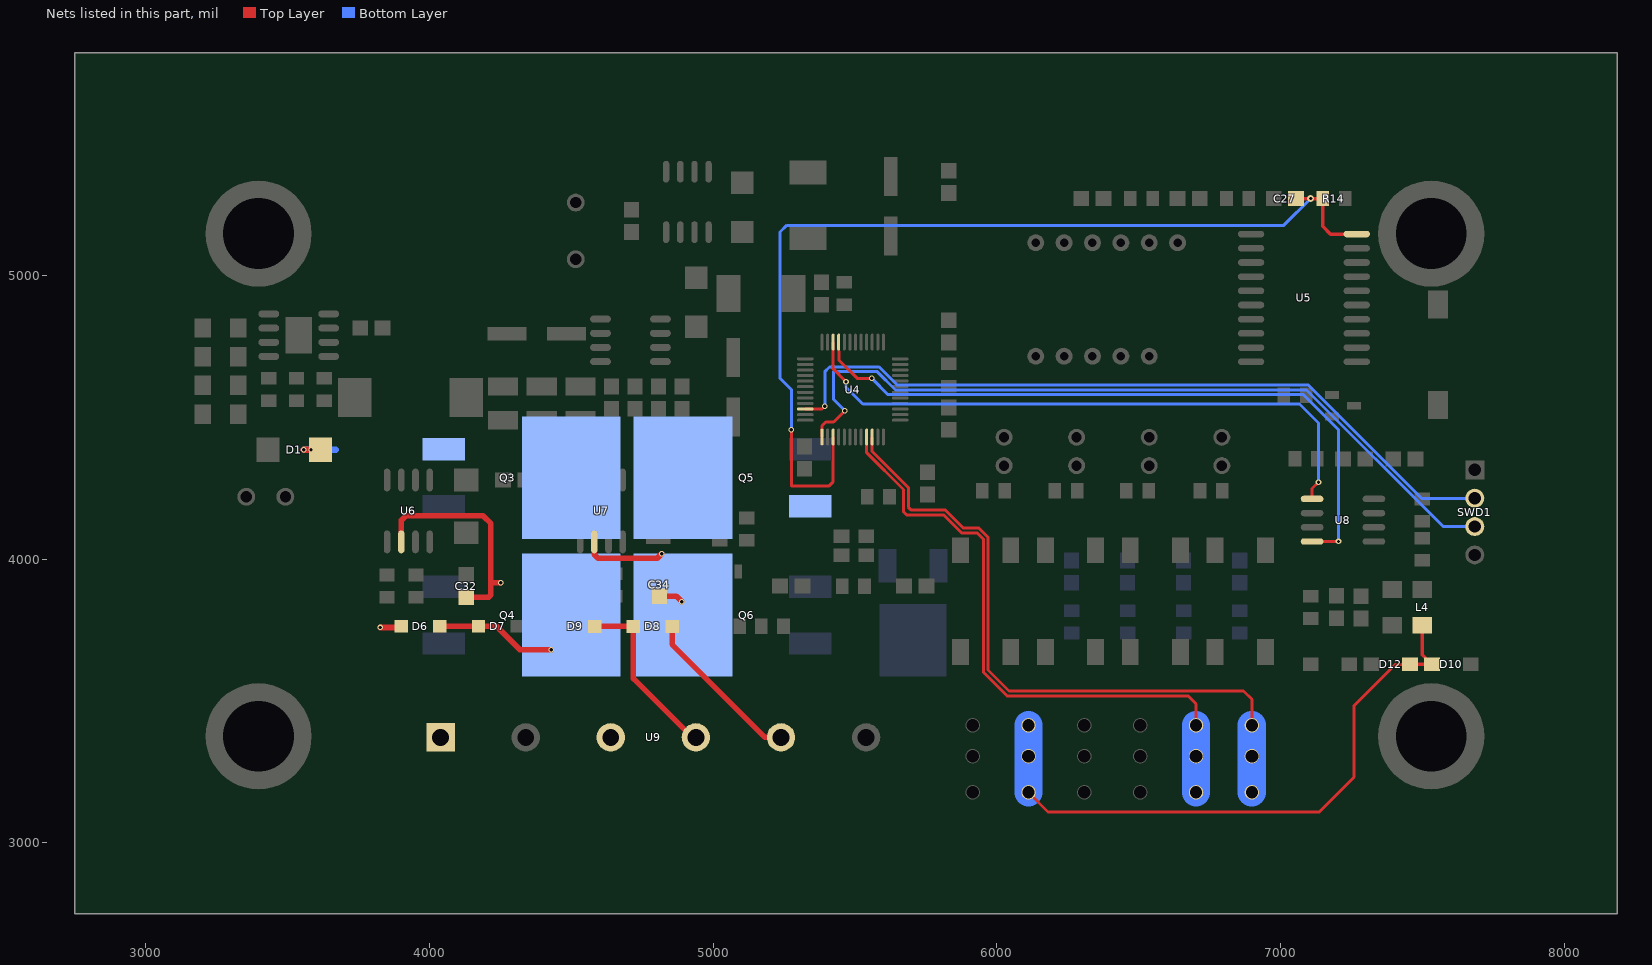
[diagram p0: the nets of this part, all layers, seen from the top]
# Altium PCB MISC82093.pcbdoc (part 2 of 2)
Units mil, origin at the board's own origin, x right, y up, seen from the top; angles counter-clockwise.
Board outline 5437 x 3035.4 mil, 2 copper layers (Top Layer, Bottom Layer), stack 62.2 mil thick; 117 components, 84 nets, 389 pads, 166 vias.

## Via types
v1: diameter 19.7, hole 11.8, Top Layer to Bottom Layer, 157 vias
v2: diameter 24, hole 12, Top Layer to Bottom Layer, 9 vias

## Nets (pads, with @x,y where several pads share a name; then routed paths per layer and width w, separated by ;. In a path a pad name is that pad's centre, name@x,y a point inside that pad or via, vN(x,y) a via of type N, cw(c..) or ccw(c..) an arc to the next point about the centre after c; other vN are vias at no path point) (continued)
RS485-B: D10.1 D12.2 L4.2 pad.0@6111.9,3178.4 pad.0@6111.9,3414.6 pad.2 | length 2202.3
  Top Layer w10.6: pad.0@6111.9,3178.4 6180.9,3109.4 7136.8,3109.4 7259.5,3232.1 7259.5,3483.9 7405.5,3629.9 D12.2@7456.8,3629.9
  Top Layer w12.5: D12.2@7456.8,3629.9 D10.1@7534.1,3629.9 7500,3664 L4.2@7500,3768
  Bottom Layer w100: pad.0@6111.9,3178.4 pad.2@6111.9,3305.9 pad.0@6111.9,3414.6
RXD: U4.22 U8.1 | length 2172.7
  Top Layer w10.6: U4.22@5423.2,4765.7 5423.2,4671.3 v1(5468.5,4626) ; U8.1@7111.5,4212.8 7111.5,4249.2 v1(7134,4271.7)
  Bottom Layer w10.6: v1(5468.5,4626) 5468.5,4606.3 5527.6,4547.2 7067.1,4547.2 7134,4480.4 v1(7134,4271.7)
S1: pad.0@6702.4,3178.4 pad.0@6702.4,3414.6 pad.3@6702.4,3305.9 U4.45 | length 2215.6
  Top Layer w10.6: U4.45@5541.3,4431.1 5541.3,4376 5671.5,4245.9 5671.5,4167.2 5682.1,4156.6 5812.5,4156.6 5876,4093.1 5930.6,4093.1 5952.5,4071.2 5952.5,3602.7 6036.4,3518.8 6674.1,3518.8 6702.4,3490.5 pad.0@6702.4,3414.6
  Bottom Layer w100: pad.0@6702.4,3178.4 pad.3@6702.4,3305.9 pad.0@6702.4,3414.6
S2: pad.0@6899.3,3178.4 pad.0@6899.3,3414.6 pad.4@6899.3,3305.9 U4.46 | length 2394
  Top Layer w10.6: U4.46@5561,4431.1 5561,4379.8 5688.1,4252.7 5688.1,4183.9 5698.7,4173.2 5819.4,4173.2 5882.9,4109.8 5937.5,4109.8 5969.2,4078.1 5969.2,3609.6 6043.3,3535.4 6870.1,3535.4 6899.3,3506.2 pad.0@6899.3,3414.6
  Bottom Layer w100: pad.0@6899.3,3178.4 pad.4@6899.3,3305.9 pad.0@6899.3,3414.6
STB: C27.1 R14.1 U4.39 U5.20 | length 3464.8
  Top Layer w10.6: v1(5275.6,4456.7) 5275.6,4259.8 5277.8,4257.7 5407.3,4257.7 5423.2,4273.6 U4.39@5423.2,4431.1
  Top Layer w12.5: C27.1@7055.1,5271.7 v2(7106.3,5271.7) R14.1@7149.2,5271.7 7149.2,5173.6 7176.6,5146.3 U5.20@7268.9,5146.3
  Bottom Layer w10.6: v1(5275.6,4456.7) 5275.6,4598.4 5236.2,4637.8 5236.2,5153.5 5259.8,5177.2 7011.8,5177.2 v2(7106.3,5271.7)
SWCLK: SWD1.3 U4.37 | length 2782.1
  Top Layer w10.6: U4.37@5383.9,4431.1 5383.9,4470.5 5397.6,4484.3 5425.2,4484.3 v1(5464.6,4523.6)
  Bottom Layer w10.6: v1(5464.6,4523.6) 5425.2,4563 5425.2,4661.4 5578.7,4661.4 5643,4597.1 7091.8,4597.1 7573.6,4115.4 SWD1.3@7685,4115.4
SWDIO: SWD1.2 U4.34 | length 2686.4
  Top Layer w10.6: U4.34@5324.8,4529.5 5383.9,4529.5 v1(5393.7,4539.4)
  Bottom Layer w10.6: v1(5393.7,4539.4) 5393.7,4661.4 5410.3,4678 5585.6,4678 5649.9,4613.8 7098.7,4613.8 7499,4213.5 7683.2,4213.5 SWD1.2@7685,4215.4
T+: C32.1 D6.2 D7.1 Q3.3 Q4.4 U6.6 U9.3 | length 1215.2
  Top Layer w20: U6.6@3900.9,4061.2 3900.9,4137.1 3917.3,4153.5 4189,4153.5 4216.5,4126 4216.5,3913.4 ; D6.2@4036.8,3763.8 D7.1@4173.2,3763.8 4236.2,3763.8 4318.9,3681.1 v1(4429.1,3681.1) ; C32.1@4129.9,3866.1 4208.7,3866.1 4216.5,3874 4216.5,3913.4 ; v1(4252,3917.3) 4220.5,3917.3 4216.5,3913.4
T-: C34.1 D8.2 D9.1 Q5.3 Q6.4 U7.6 U9.4 | length 1006.9
  Top Layer w20: U7.6@4581.3,4061.2 4581.3,4017.1 4594.5,4003.9 4803.1,4003.9 v1(4818.9,4019.7) ; D9.1@4582.7,3763.5 D8.2@4719.1,3763.5 4719.1,3580.1 4927,3372.2 U9.4@4939.4,3372.2 ; C34.1@4811,3870.1 4870.1,3870.1 v1(4889.8,3850.4)
TXD: U4.21 U8.4 | length 2413.6
  Top Layer w10.6: U4.21@5442.9,4765.7 5443,4702.7 5507.9,4637.8 v1(5559.1,4637.8) ; U8.4@7111.5,4062.8 7111.7,4063 v1(7204.7,4063)
  Bottom Layer w10.6: v1(5559.1,4637.8) 5616.3,4580.5 7080.9,4580.5 7204.7,4456.7 v1(7204.7,4063)
VCC: D1.2 D6.1 D8.1 Q3.4 Q5.4 U9.1 U9.5 | length 847.6
  Top Layer w20: v1(3826.8,3759.8) 3896.3,3759.8 D6.1@3900.2,3763.8 ; D8.1@4855.7,3763.5 4855.7,3699.4 5182.9,3372.2 U9.5@5239.4,3372.2
  Top Layer w23.6: v1(3557,4385.8) v1(3582.8,4385.8) D1.2@3633.9,4385.8
  Bottom Layer w23.6: v1(3557,4385.8) v1(3582.8,4385.8) 3669.3,4385.8
pads on no net: SW1.2 SW2.2 SW3.2 SW4.2 U1.6 U4.2 U4.3 U4.4 U4.19 U4.25 U4.26 U4.29 U4.33 U4.38 U5.10 U5.11 U5.13
copper on no net:
  other v1: 3366.2,3228.4 3429,3228.4 7500.1,3228.4 7562.9,3228.4 3308.9,3254 3486.4,3254 7442.7,3254 7620.3,3254 3266.9,3300.6 3528.4,3300.6 7400.7,3300.6 7662.3,3300.6 3247.5,3360.4 3547.8,3360.4 7381.3,3360.4 7681.7,3360.4 3254,3422.8 3541.3,3422.8 7387.9,3422.8 7675.1,3422.8 3285.4,3477.2 3509.9,3477.2 7419.3,3477.2 7643.7,3477.2 3336.2,3514.1 3459.1,3514.1 7470.1,3514.1 7592.9,3514.1 3397.6,3527.1 7531.5,3527.1 3366.2,5000.1 3429,5000.1 7500.1,5000.1 7562.9,5000.1 3308.9,5025.6 3486.4,5025.6 7442.7,5025.6 7620.3,5025.6 3266.9,5072.3 3528.4,5072.3 7400.7,5072.3 7662.3,5072.3 3247.5,5132 3547.8,5132 7381.3,5132 7681.7,5132 3254,5194.5 3541.3,5194.5 7387.9,5194.5 7675.1,5194.5 3285.4,5248.8 3509.9,5248.8 7419.3,5248.8 7643.7,5248.8 3336.2,5285.7 3459.1,5285.7 7470.1,5285.7 7592.9,5285.7 3397.6,5298.8 7531.5,5298.8

## Polygon pours and split planes (outlines as drawn)
VCC on Top Layer (solid, remove dead copper, pour order 6): 4137.8,3543.3 4179.8,3501.3 4179.8,3100.6 4150.1,3070.9 3858.3,3070.9 3858.3,3543.3
GND on Top Layer (solid, remove dead copper, pour order 10): 3019.7,5523.6 3019.7,3000 7905.5,3000 7905.5,5523.6
VCC on Bottom Layer (solid, remove dead copper, pour order 24): 4317.2,4051.2 4281.8,4086.6 4281.8,4525.3 4267.7,4539.4 3908.6,4539.4 3874,4504.8 3874,3547.2 3913.4,3507.9 4137.8,3507.9 4161.4,3484.3 4161.4,3255.9 4133.9,3228.3 3641.7,3228.3 3618.1,3252 3618.1,4752 3673.2,4807.1 5070.9,4807.1 5110.2,4767.7 5110.2,4063 5098.4,4051.2
T+ on Bottom Layer (solid, remove dead copper, pour order 26): 4511.8,3232.3 4496.1,3248 4496.1,3468.5 4437,3527.6 4354.3,3527.6 4205.3,3676.6 4205.3,3987.3 4180.8,4011.8 3893.7,4011.8 3877.8,4027.7 3877.8,4504.8 3910.9,4537.9 4247.9,4537.9 4275.6,4510.2 4275.6,4080.4 4308.8,4047.2 4673.2,4047.2 4692.9,4027.6 4692.9,3559.1 4779.7,3472.2 4779.7,3250.2 4761.8,3232.3
T- on Bottom Layer (solid, remove dead copper, pour order 28): 4791.3,3468.5 4696.9,3563 4696.9,4031.5 4712.6,4047.2 5098.4,4047.2 5113.5,4062.3 5113.5,4148.9 5114.2,4149.6 5114.2,4259.8 5129.9,4275.6 5437.2,4275.6 5453,4259.8 5453,4008.1 5440.9,3996.1 5255.9,3996.1 5236.2,3976.4 5236.2,3645.7 5063,3472.4 5063,3252 5043.8,3232.8 4806.6,3232.8 4791.3,3248
VCC on Top Layer (solid, remove dead copper, pour order 8): 5102.4,3476.4 5326.8,3476.4 5358.3,3444.9 5358.3,3102.4 5334.6,3078.7 4141.7,3078.7 4118.1,3102.4 4118.1,3263.8 4145.7,3291.3 5051.2,3291.3 5078.7,3318.9 5078.7,3452.8
GND on Bottom Layer (solid, remove dead copper, pour order 30): 3000,5535.4 3000,3000 7937,3000 7937,5535.4

## Keep-outs
Top Layer:
  region: 3594.5,5147.8 3594.1,5135.3 3592.9,5122.9 3590.9,5110.5 3588.2,5098.4 3584.7,5086.4 3580.4,5074.6 3575.4,5063.2 3569.7,5052.1 3563.2,5041.4 3556.2,5031.1 3548.4,5021.3 3540.1,5012 3531.2,5003.2 3521.8,4995 3511.8,4987.4 3501.4,4980.5 3490.6,4974.3 3479.4,4968.7 3467.9,4963.9 3456.1,4959.8 3444,4956.5 3431.8,4953.9 3419.5,4952.2 3407,4951.2 3394.5,4951 3382,4951.6 3369.6,4952.9 3357.3,4955.1 3345.2,4958.1 3333.3,4961.8 3321.6,4966.2 3310.2,4971.4 3299.2,4977.3 3288.6,4983.9 3278.4,4991.1 3268.7,4999 3259.6,5007.5 3250.9,5016.5 3242.9,5026.1 3235.5,5036.2 3228.7,5046.7 3222.7,5057.6 3217.3,5068.9 3212.7,5080.5 3208.8,5092.3 3205.6,5104.4 3203.3,5116.7 3201.7,5129.1 3200.9,5141.5 3200.9,5154 3201.7,5166.5 3203.3,5178.9 3205.6,5191.2 3208.8,5203.3 3212.7,5215.1 3217.3,5226.7 3222.7,5238 3228.7,5248.9 3235.5,5259.4 3242.9,5269.5 3250.9,5279 3259.6,5288.1 3268.7,5296.6 3278.4,5304.4 3288.6,5311.7 3299.2,5318.3 3310.2,5324.2 3321.6,5329.4 3333.3,5333.8 3345.2,5337.5 3357.3,5340.5 3369.6,5342.6 3382,5344 3394.5,5344.6 3407,5344.4 3419.5,5343.4 3431.8,5341.7 3444,5339.1 3456.1,5335.8 3467.9,5331.7 3479.4,5326.9 3490.6,5321.3 3501.4,5315.1 3511.8,5308.1 3521.8,5300.6 3531.2,5292.4 3540.1,5283.6 3548.4,5274.3 3556.2,5264.5 3563.2,5254.2 3569.7,5243.5 3575.4,5232.4 3580.4,5221 3584.7,5209.2 3588.2,5197.2 3590.9,5185 3592.9,5172.7 3594.1,5160.3
  region: 3594.5,3376.1 3594.1,3363.7 3592.9,3351.2 3590.9,3338.9 3588.2,3326.7 3584.7,3314.7 3580.4,3303 3575.4,3291.5 3569.7,3280.4 3563.2,3269.7 3556.2,3259.4 3548.4,3249.6 3540.1,3240.3 3531.2,3231.5 3521.8,3223.4 3511.8,3215.8 3501.4,3208.9 3490.6,3202.6 3479.4,3197.1 3467.9,3192.3 3456.1,3188.2 3444,3184.8 3431.8,3182.3 3419.5,3180.5 3407,3179.5 3394.5,3179.3 3382,3179.9 3369.6,3181.3 3357.3,3183.5 3345.2,3186.4 3333.3,3190.1 3321.6,3194.6 3310.2,3199.8 3299.2,3205.7 3288.6,3212.3 3278.4,3219.5 3268.7,3227.4 3259.6,3235.8 3250.9,3244.9 3242.9,3254.5 3235.5,3264.5 3228.7,3275 3222.7,3285.9 3217.3,3297.2 3212.7,3308.8 3208.8,3320.7 3205.6,3332.8 3203.3,3345 3201.7,3357.4 3200.9,3369.9 3200.9,3382.4 3201.7,3394.9 3203.3,3407.2 3205.6,3419.5 3208.8,3431.6 3212.7,3443.5 3217.3,3455.1 3222.7,3466.3 3228.7,3477.3 3235.5,3487.8 3242.9,3497.8 3250.9,3507.4 3259.6,3516.4 3268.7,3524.9 3278.4,3532.8 3288.6,3540 3299.2,3546.6 3310.2,3552.5 3321.6,3557.7 3333.3,3562.2 3345.2,3565.9 3357.3,3568.8 3369.6,3571 3382,3572.4 3394.5,3573 3407,3572.8 3419.5,3571.8 3431.8,3570 3444,3567.4 3456.1,3564.1 3467.9,3560 3479.4,3555.2 3490.6,3549.7 3501.4,3543.4 3511.8,3536.5 3521.8,3528.9 3531.2,3520.7 3540.1,3512 3548.4,3502.7 3556.2,3492.9 3563.2,3482.6 3569.7,3471.8 3575.4,3460.7 3580.4,3449.3 3584.7,3437.6 3588.2,3425.6 3590.9,3413.4 3592.9,3401.1 3594.1,3388.6
  region: 7728.3,3376.1 7728,3363.7 7726.8,3351.2 7724.8,3338.9 7722,3326.7 7718.5,3314.7 7714.2,3303 7709.2,3291.5 7703.5,3280.4 7697.1,3269.7 7690,3259.4 7682.3,3249.6 7674,3240.3 7665.1,3231.5 7655.6,3223.4 7645.7,3215.8 7635.3,3208.9 7624.5,3202.6 7613.3,3197.1 7601.7,3192.3 7589.9,3188.2 7577.9,3184.8 7565.7,3182.3 7553.3,3180.5 7540.9,3179.5 7528.4,3179.3 7515.9,3179.9 7503.5,3181.3 7491.2,3183.5 7479,3186.4 7467.1,3190.1 7455.4,3194.6 7444.1,3199.8 7433.1,3205.7 7422.5,3212.3 7412.3,3219.5 7402.6,3227.4 7393.4,3235.8 7384.8,3244.9 7376.8,3254.5 7369.4,3264.5 7362.6,3275 7356.5,3285.9 7351.2,3297.2 7346.5,3308.8 7342.6,3320.7 7339.5,3332.8 7337.1,3345 7335.5,3357.4 7334.7,3369.9 7334.7,3382.4 7335.5,3394.9 7337.1,3407.2 7339.5,3419.5 7342.6,3431.6 7346.5,3443.5 7351.2,3455.1 7356.5,3466.3 7362.6,3477.3 7369.4,3487.8 7376.8,3497.8 7384.8,3507.4 7393.4,3516.4 7402.6,3524.9 7412.3,3532.8 7422.5,3540 7433.1,3546.6 7444.1,3552.5 7455.4,3557.7 7467.1,3562.2 7479,3565.9 7491.2,3568.8 7503.5,3571 7515.9,3572.4 7528.4,3573 7540.9,3572.8 7553.3,3571.8 7565.7,3570 7577.9,3567.4 7589.9,3564.1 7601.7,3560 7613.3,3555.2 7624.5,3549.7 7635.3,3543.4 7645.7,3536.5 7655.6,3528.9 7665.1,3520.7 7674,3512 7682.3,3502.7 7690,3492.9 7697.1,3482.6 7703.5,3471.8 7709.2,3460.7 7714.2,3449.3 7718.5,3437.6 7722,3425.6 7724.8,3413.4 7726.8,3401.1 7728,3388.6
  region: 7728.3,5147.8 7728,5135.3 7726.8,5122.9 7724.8,5110.5 7722,5098.4 7718.5,5086.4 7714.2,5074.6 7709.2,5063.2 7703.5,5052.1 7697.1,5041.4 7690,5031.1 7682.3,5021.3 7674,5012 7665.1,5003.2 7655.6,4995 7645.7,4987.4 7635.3,4980.5 7624.5,4974.3 7613.3,4968.7 7601.7,4963.9 7589.9,4959.8 7577.9,4956.5 7565.7,4953.9 7553.3,4952.2 7540.9,4951.2 7528.4,4951 7515.9,4951.6 7503.5,4952.9 7491.2,4955.1 7479,4958.1 7467.1,4961.8 7455.4,4966.2 7444.1,4971.4 7433.1,4977.3 7422.5,4983.9 7412.3,4991.1 7402.6,4999 7393.4,5007.5 7384.8,5016.5 7376.8,5026.1 7369.4,5036.2 7362.6,5046.7 7356.5,5057.6 7351.2,5068.9 7346.5,5080.5 7342.6,5092.3 7339.5,5104.4 7337.1,5116.7 7335.5,5129.1 7334.7,5141.5 7334.7,5154 7335.5,5166.5 7337.1,5178.9 7339.5,5191.2 7342.6,5203.3 7346.5,5215.1 7351.2,5226.7 7356.5,5238 7362.6,5248.9 7369.4,5259.4 7376.8,5269.5 7384.8,5279 7393.4,5288.1 7402.6,5296.6 7412.3,5304.4 7422.5,5311.7 7433.1,5318.3 7444.1,5324.2 7455.4,5329.4 7467.1,5333.8 7479,5337.5 7491.2,5340.5 7503.5,5342.6 7515.9,5344 7528.4,5344.6 7540.9,5344.4 7553.3,5343.4 7565.7,5341.7 7577.9,5339.1 7589.9,5335.8 7601.7,5331.7 7613.3,5326.9 7624.5,5321.3 7635.3,5315.1 7645.7,5308.1 7655.6,5300.6 7665.1,5292.4 7674,5283.6 7682.3,5274.3 7690,5264.5 7697.1,5254.2 7703.5,5243.5 7709.2,5232.4 7714.2,5221 7718.5,5209.2 7722,5197.2 7724.8,5185 7726.8,5172.7 7728,5160.3
Bottom Layer:
  region: 7728.3,5147.8 7728,5135.3 7726.8,5122.9 7724.8,5110.5 7722,5098.4 7718.5,5086.4 7714.2,5074.6 7709.2,5063.2 7703.5,5052.1 7697.1,5041.4 7690,5031.1 7682.3,5021.3 7674,5012 7665.1,5003.2 7655.6,4995 7645.7,4987.4 7635.3,4980.5 7624.5,4974.3 7613.3,4968.7 7601.7,4963.9 7589.9,4959.8 7577.9,4956.5 7565.7,4953.9 7553.3,4952.2 7540.9,4951.2 7528.4,4951 7515.9,4951.6 7503.5,4952.9 7491.2,4955.1 7479,4958.1 7467.1,4961.8 7455.4,4966.2 7444.1,4971.4 7433.1,4977.3 7422.5,4983.9 7412.3,4991.1 7402.6,4999 7393.4,5007.5 7384.8,5016.5 7376.8,5026.1 7369.4,5036.2 7362.6,5046.7 7356.5,5057.6 7351.2,5068.9 7346.5,5080.5 7342.6,5092.3 7339.5,5104.4 7337.1,5116.7 7335.5,5129.1 7334.7,5141.5 7334.7,5154 7335.5,5166.5 7337.1,5178.9 7339.5,5191.2 7342.6,5203.3 7346.5,5215.1 7351.2,5226.7 7356.5,5238 7362.6,5248.9 7369.4,5259.4 7376.8,5269.5 7384.8,5279 7393.4,5288.1 7402.6,5296.6 7412.3,5304.4 7422.5,5311.7 7433.1,5318.3 7444.1,5324.2 7455.4,5329.4 7467.1,5333.8 7479,5337.5 7491.2,5340.5 7503.5,5342.6 7515.9,5344 7528.4,5344.6 7540.9,5344.4 7553.3,5343.4 7565.7,5341.7 7577.9,5339.1 7589.9,5335.8 7601.7,5331.7 7613.3,5326.9 7624.5,5321.3 7635.3,5315.1 7645.7,5308.1 7655.6,5300.6 7665.1,5292.4 7674,5283.6 7682.3,5274.3 7690,5264.5 7697.1,5254.2 7703.5,5243.5 7709.2,5232.4 7714.2,5221 7718.5,5209.2 7722,5197.2 7724.8,5185 7726.8,5172.7 7728,5160.3
  region: 7728.3,3376.1 7728,3363.7 7726.8,3351.2 7724.8,3338.9 7722,3326.7 7718.5,3314.7 7714.2,3303 7709.2,3291.5 7703.5,3280.4 7697.1,3269.7 7690,3259.4 7682.3,3249.6 7674,3240.3 7665.1,3231.5 7655.6,3223.4 7645.7,3215.8 7635.3,3208.9 7624.5,3202.6 7613.3,3197.1 7601.7,3192.3 7589.9,3188.2 7577.9,3184.8 7565.7,3182.3 7553.3,3180.5 7540.9,3179.5 7528.4,3179.3 7515.9,3179.9 7503.5,3181.3 7491.2,3183.5 7479,3186.4 7467.1,3190.1 7455.4,3194.6 7444.1,3199.8 7433.1,3205.7 7422.5,3212.3 7412.3,3219.5 7402.6,3227.4 7393.4,3235.8 7384.8,3244.9 7376.8,3254.5 7369.4,3264.5 7362.6,3275 7356.5,3285.9 7351.2,3297.2 7346.5,3308.8 7342.6,3320.7 7339.5,3332.8 7337.1,3345 7335.5,3357.4 7334.7,3369.9 7334.7,3382.4 7335.5,3394.9 7337.1,3407.2 7339.5,3419.5 7342.6,3431.6 7346.5,3443.5 7351.2,3455.1 7356.5,3466.3 7362.6,3477.3 7369.4,3487.8 7376.8,3497.8 7384.8,3507.4 7393.4,3516.4 7402.6,3524.9 7412.3,3532.8 7422.5,3540 7433.1,3546.6 7444.1,3552.5 7455.4,3557.7 7467.1,3562.2 7479,3565.9 7491.2,3568.8 7503.5,3571 7515.9,3572.4 7528.4,3573 7540.9,3572.8 7553.3,3571.8 7565.7,3570 7577.9,3567.4 7589.9,3564.1 7601.7,3560 7613.3,3555.2 7624.5,3549.7 7635.3,3543.4 7645.7,3536.5 7655.6,3528.9 7665.1,3520.7 7674,3512 7682.3,3502.7 7690,3492.9 7697.1,3482.6 7703.5,3471.8 7709.2,3460.7 7714.2,3449.3 7718.5,3437.6 7722,3425.6 7724.8,3413.4 7726.8,3401.1 7728,3388.6
  region: 3594.5,3376.1 3594.1,3363.7 3592.9,3351.2 3590.9,3338.9 3588.2,3326.7 3584.7,3314.7 3580.4,3303 3575.4,3291.5 3569.7,3280.4 3563.2,3269.7 3556.2,3259.4 3548.4,3249.6 3540.1,3240.3 3531.2,3231.5 3521.8,3223.4 3511.8,3215.8 3501.4,3208.9 3490.6,3202.6 3479.4,3197.1 3467.9,3192.3 3456.1,3188.2 3444,3184.8 3431.8,3182.3 3419.5,3180.5 3407,3179.5 3394.5,3179.3 3382,3179.9 3369.6,3181.3 3357.3,3183.5 3345.2,3186.4 3333.3,3190.1 3321.6,3194.6 3310.2,3199.8 3299.2,3205.7 3288.6,3212.3 3278.4,3219.5 3268.7,3227.4 3259.6,3235.8 3250.9,3244.9 3242.9,3254.5 3235.5,3264.5 3228.7,3275 3222.7,3285.9 3217.3,3297.2 3212.7,3308.8 3208.8,3320.7 3205.6,3332.8 3203.3,3345 3201.7,3357.4 3200.9,3369.9 3200.9,3382.4 3201.7,3394.9 3203.3,3407.2 3205.6,3419.5 3208.8,3431.6 3212.7,3443.5 3217.3,3455.1 3222.7,3466.3 3228.7,3477.3 3235.5,3487.8 3242.9,3497.8 3250.9,3507.4 3259.6,3516.4 3268.7,3524.9 3278.4,3532.8 3288.6,3540 3299.2,3546.6 3310.2,3552.5 3321.6,3557.7 3333.3,3562.2 3345.2,3565.9 3357.3,3568.8 3369.6,3571 3382,3572.4 3394.5,3573 3407,3572.8 3419.5,3571.8 3431.8,3570 3444,3567.4 3456.1,3564.1 3467.9,3560 3479.4,3555.2 3490.6,3549.7 3501.4,3543.4 3511.8,3536.5 3521.8,3528.9 3531.2,3520.7 3540.1,3512 3548.4,3502.7 3556.2,3492.9 3563.2,3482.6 3569.7,3471.8 3575.4,3460.7 3580.4,3449.3 3584.7,3437.6 3588.2,3425.6 3590.9,3413.4 3592.9,3401.1 3594.1,3388.6
  region: 3594.5,5147.8 3594.1,5135.3 3592.9,5122.9 3590.9,5110.5 3588.2,5098.4 3584.7,5086.4 3580.4,5074.6 3575.4,5063.2 3569.7,5052.1 3563.2,5041.4 3556.2,5031.1 3548.4,5021.3 3540.1,5012 3531.2,5003.2 3521.8,4995 3511.8,4987.4 3501.4,4980.5 3490.6,4974.3 3479.4,4968.7 3467.9,4963.9 3456.1,4959.8 3444,4956.5 3431.8,4953.9 3419.5,4952.2 3407,4951.2 3394.5,4951 3382,4951.6 3369.6,4952.9 3357.3,4955.1 3345.2,4958.1 3333.3,4961.8 3321.6,4966.2 3310.2,4971.4 3299.2,4977.3 3288.6,4983.9 3278.4,4991.1 3268.7,4999 3259.6,5007.5 3250.9,5016.5 3242.9,5026.1 3235.5,5036.2 3228.7,5046.7 3222.7,5057.6 3217.3,5068.9 3212.7,5080.5 3208.8,5092.3 3205.6,5104.4 3203.3,5116.7 3201.7,5129.1 3200.9,5141.5 3200.9,5154 3201.7,5166.5 3203.3,5178.9 3205.6,5191.2 3208.8,5203.3 3212.7,5215.1 3217.3,5226.7 3222.7,5238 3228.7,5248.9 3235.5,5259.4 3242.9,5269.5 3250.9,5279 3259.6,5288.1 3268.7,5296.6 3278.4,5304.4 3288.6,5311.7 3299.2,5318.3 3310.2,5324.2 3321.6,5329.4 3333.3,5333.8 3345.2,5337.5 3357.3,5340.5 3369.6,5342.6 3382,5344 3394.5,5344.6 3407,5344.4 3419.5,5343.4 3431.8,5341.7 3444,5339.1 3456.1,5335.8 3467.9,5331.7 3479.4,5326.9 3490.6,5321.3 3501.4,5315.1 3511.8,5308.1 3521.8,5300.6 3531.2,5292.4 3540.1,5283.6 3548.4,5274.3 3556.2,5264.5 3563.2,5254.2 3569.7,5243.5 3575.4,5232.4 3580.4,5221 3584.7,5209.2 3588.2,5197.2 3590.9,5185 3592.9,5172.7 3594.1,5160.3
Board Outline Layer:
  region: 3248.1,4148.4 3248.1,3612.3 3598.7,3612.3 3598.7,4148.4
  region: 3248.1,4148.4 3248.1,3612.3 3598.7,3612.3 3598.7,4148.4
  lines w0.1: 3248.1,3612.3 3248.1,4148.4 3598.7,4148.4 3598.7,3612.3 3248.1,3612.3
  lines w3.9: 3102.4,3267.7 3102.4,5236.2 3102.8,5248.6 3103.9,5260.9 3105.8,5273.1 3108.5,5285.2 3112,5297.1 3116.2,5308.7 3121.1,5320 3126.7,5331.1 3133,5341.7 3140,5351.9 3147.5,5361.7 3155.7,5371 3164.5,5379.7 3173.7,5387.9 3183.5,5395.5 3193.7,5402.4 3204.4,5408.7 3215.4,5414.3 3226.7,5419.2 3238.4,5423.4 3250.3,5426.9 3262.3,5429.6 3274.5,5431.5 3286.9,5432.7 3299.2,5433.1 3717.7,5433.1 3722.8,5432.7 3727.9,5431.7 3732.7,5430.1 3737.4,5427.8 3741.6,5424.9 3745.5,5421.5 3748.9,5417.7 3751.8,5413.4 3754,5408.8 3755.7,5403.9 3756.7,5398.8 3757,5393.7 3757,4968.5 3757.4,4963.4 3758.4,4958.3 3760,4953.4 3762.3,4948.8 3765.2,4944.5 3768.6,4940.7 3772.4,4937.3 3776.7,4934.4 3781.3,4932.1 3786.2,4930.5 3791.3,4929.5 3796.4,4929.1 4345.5,4929.1 4350.7,4929.5 4355.7,4930.5 4360.6,4932.1 4365.2,4934.4 4369.5,4937.3 4373.4,4940.7 4376.8,4944.5 4379.6,4948.8 4381.9,4953.4 4383.5,4958.3 4384.6,4963.4 4384.9,4968.5 4384.9,5393.8 4385.2,5398.9 4386.2,5404 4387.9,5408.8 4390.2,5413.5 4393,5417.7 4396.4,5421.6 4400.3,5425 4404.6,5427.9 4409.2,5430.1 4414.1,5431.8 4419.1,5432.8 4424.3,5433.1 7629.9,5433.1 7642.3,5432.7 7654.6,5431.5 7666.8,5429.6 7678.9,5426.9 7690.8,5423.4 7702.4,5419.2 7713.7,5414.3 7724.8,5408.7 7735.4,5402.4 7745.6,5395.5 7755.4,5387.9 7764.7,5379.7 7773.4,5371 7781.6,5361.7 7789.2,5351.9 7796.1,5341.7 7802.4,5331.1 7808,5320 7812.9,5308.7 7817.1,5297.1 7820.6,5285.2 7823.3,5273.1 7825.2,5260.9 7826.4,5248.6 7826.8,5236.2 7826.8,3267.7 7826.4,3255.4 7825.2,3243 7823.3,3230.8 7820.6,3218.8 7817.1,3206.9 7812.9,3195.3 7808,3183.9 7802.4,3172.9 7796.1,3162.2 7789.2,3152 7781.6,3142.2 7773.4,3133 7764.7,3124.2 7755.4,3116 7745.6,3108.5 7735.4,3101.5 7724.8,3095.2 7713.7,3089.6 7702.4,3084.7 7690.8,3080.5 7678.9,3077.1 7666.8,3074.4 7654.6,3072.4 7642.3,3071.3 7629.9,3070.9 3299.2,3070.9 3286.9,3071.3 3274.5,3072.4 3262.3,3074.4 3250.3,3077.1 3238.4,3080.5 3226.7,3084.7 3215.4,3089.6 3204.4,3095.2 3193.7,3101.5 3183.5,3108.5 3173.7,3116 3164.5,3124.2 3155.7,3133 3147.5,3142.2 3140,3152 3133,3162.2 3126.7,3172.9 3121.1,3183.9 3116.2,3195.3 3112,3206.9 3108.5,3218.8 3105.8,3230.8 3103.9,3243 3102.8,3255.4 3102.4,3267.7

## Other copper
Top Layer:
  drawing of 314 lines, arcs and shapes, not listed
Bottom Layer:
  region net K1: 6221.3,3911.9 6221.3,3922.5 6224.9,3922.9 6228.5,3923.9 6231.8,3925.5 6234.7,3927.8 6237.2,3930.5 6237.2,3903.9 6234.7,3906.7 6231.8,3908.9 6228.5,3910.6 6224.9,3911.6 6221.3,3911.9
  region net K2: 6418.8,3911.9 6418.8,3922.5 6422.5,3922.9 6426.1,3923.9 6429.4,3925.5 6432.3,3927.8 6434.8,3930.5 6434.8,3903.9 6432.3,3906.7 6429.4,3908.9 6426.1,3910.6 6422.5,3911.6 6418.8,3911.9
  region net K3: 6616.4,3911.9 6616.4,3922.5 6620.1,3922.9 6623.6,3923.9 6626.9,3925.5 6629.9,3927.8 6632.4,3930.5 6632.4,3903.9 6629.9,3906.7 6626.9,3908.9 6623.6,3910.6 6620.1,3911.6 6616.4,3911.9
  region net K4: 6899,3922.5 6899,3911.9 6895.4,3911.6 6891.8,3910.6 6888.5,3908.9 6885.6,3906.7 6883.1,3903.9 6883.1,3930.5 6885.6,3927.8 6888.5,3925.5 6891.8,3923.9 6895.4,3922.9 6899,3922.5
  region net FAN-: 5754.7,3537.6 5654.7,3537.6 5652,3544.5 5648.6,3551.2 5644.5,3557.5 5639.8,3563.3 5634.5,3568.6 5628.7,3573.3 5622.4,3577.3 5615.7,3580.7 5608.7,3583.4 5601.5,3585.3 5594.1,3586.5 5586.6,3586.9 5822.8,3586.9 5815.4,3586.5 5808,3585.3 5800.7,3583.4 5793.7,3580.7 5787.1,3577.3 5780.8,3573.3 5775,3568.6 5769.7,3563.3 5764.9,3557.5 5760.8,3551.2 5757.4,3544.5 5754.7,3537.6
  region net $1N21282: 5553.3,3968.1 5553.3,3988.1 5558.2,3988.4 5563.1,3989.4 5567.8,3991 5572.2,3993.2 5576.3,3996 5580,3999.3 5583.3,4003.1 5583.3,3953.1 5580,3956.8 5576.3,3960.1 5572.2,3962.9 5567.8,3965.1 5563.1,3966.7 5558.2,3967.7 5553.3,3968.1
  region net $1N16482: 6220.7,3734.7 6220.7,3745.4 6224.4,3745.7 6228,3746.7 6231.3,3748.4 6234.2,3750.6 6236.7,3753.3 6236.7,3726.8 6234.2,3729.5 6231.3,3731.7 6228,3733.4 6224.4,3734.4 6220.7,3734.7
  region net +3.3V: 6320.9,3828.8 6320.9,3808.8 6315.4,3808.4 6309.9,3807.4 6304.7,3805.6 6299.7,3803.2 6295.1,3800.1 6290.9,3796.5 6290.9,3841.1 6295.1,3837.5 6299.7,3834.4 6304.7,3832 6309.9,3830.2 6315.4,3829.2 6320.9,3828.8
  region net $1N16483: 6465.9,3701.8 6455.3,3701.8 6455,3705.5 6454,3709 6452.3,3712.3 6450.1,3715.3 6447.3,3717.8 6473.9,3717.8 6471.2,3715.3 6469,3712.3 6467.3,3709 6466.3,3705.5 6465.9,3701.8
  region net +3.3V: 6404.3,3808.8 6404.2,3828.8 6409.8,3829.2 6415.2,3830.2 6420.5,3832 6425.4,3834.4 6430.1,3837.5 6434.3,3841.1 6434.2,3796.5 6430.1,3800.1 6425.4,3803.2 6420.5,3805.6 6415.2,3807.4 6409.8,3808.4 6404.2,3808.8
  region net +3.3V: 6518.5,3828.8 6518.5,3808.8 6512.9,3808.5 6507.5,3807.4 6502.2,3805.6 6497.3,3803.2 6492.6,3800.1 6488.5,3796.5 6488.5,3841.1 6492.7,3837.5 6497.3,3834.4 6502.3,3832 6507.5,3830.3 6512.9,3829.2
  region net $1N16484: 6666.7,3701.8 6656.1,3701.8 6655.8,3705.5 6654.7,3709 6653.1,3712.3 6650.9,3715.3 6648.1,3717.8 6674.7,3717.8 6672,3715.3 6669.7,3712.3 6668.1,3709 6667.1,3705.5 6666.7,3701.8
  region net +3.3V: 6601.8,3808.9 6601.8,3828.9 6607.4,3829.2 6612.8,3830.3 6618,3832 6623,3834.5 6627.6,3837.5 6631.8,3841.1 6631.8,3796.5 6627.6,3800.2 6623,3803.2 6618,3805.7 6612.8,3807.4 6607.4,3808.5 6601.8,3808.9
  region net +3.3V: 6716,3828.9 6716,3808.9 6710.5,3808.5 6705.1,3807.5 6699.8,3805.7 6694.8,3803.2 6690.2,3800.2 6686,3796.5 6686,3841.1 6690.2,3837.5 6694.9,3834.5 6699.8,3832.1 6705.1,3830.3 6710.5,3829.3 6716,3828.9
  region net $1N16495: 6861.8,3701.8 6851.2,3701.8 6850.9,3705.5 6849.8,3709 6848.2,3712.3 6846,3715.3 6843.2,3717.8 6869.8,3717.8 6867.1,3715.3 6864.8,3712.3 6863.2,3709 6862.2,3705.5 6861.8,3701.8
  region net +3.3V: 6799.4,3808.9 6799.4,3828.9 6804.9,3829.3 6810.3,3830.3 6815.6,3832.1 6820.6,3834.5 6825.2,3837.5 6829.4,3841.1 6829.4,3796.5 6825.2,3800.2 6820.6,3803.2 6815.6,3805.7 6810.4,3807.5 6804.9,3808.5 6799.4,3808.9
  region net +3.3V: 6913.6,3828.9 6913.6,3808.9 6908.1,3808.5 6902.6,3807.5 6897.4,3805.7 6892.4,3803.2 6887.8,3800.2 6883.6,3796.5 6883.6,3841.1 6887.8,3837.5 6892.4,3834.5 6897.4,3832.1 6902.7,3830.3 6908.1,3829.3 6913.6,3828.9
  region net SWDIO: 7640.9,4208.2 7638.1,4218.8 7639.1,4219.3 7640.9,4220.5 7646.5,4225.2 7653.7,4231.7 7661.5,4239.2 7664.3,4189.1 7662.4,4191 7660,4193.6 7657.3,4196.7 7654.4,4200 7651.2,4203.1 7649.5,4204.5 7647.9,4205.7 7646.2,4206.7 7644.4,4207.5 7642.7,4208
  region net SWCLK: 7639.5,4110 7639.5,4120.7 7641.8,4122.4 7647.2,4126.9 7662.9,4140.5 7662.9,4090.3 7647.2,4103.9 7641.8,4108.3
  region net E: 6131.5,4757 6144.1,4756.4 6144.4,4755.5 6145.4,4754 6149.1,4749 6154.2,4742.5 6160.1,4735.4 6115.2,4736 6121.2,4742.9 6126.4,4749.4 6130.1,4754.4 6131.2,4756.1
  region net D: 6230,4755.8 6242.5,4757.6 6242.9,4756.5 6243.9,4754.7 6247.7,4749.7 6253,4743.3 6259.1,4736.6 6214.1,4734.8 6219.9,4742.1 6225,4748.7 6228.6,4753.6 6229.6,4755.1
  region net C: 6430.7,4756.4 6443.3,4757 6443.6,4756 6444.7,4754.4 6448.4,4749.3 6453.6,4742.9 6459.6,4736 6414.6,4735.4 6420.5,4742.5 6425.7,4749 6429.4,4754 6430.4,4755.6
  region net B: 6644.1,5075.4 6631.5,5074.7 6631.2,5075.7 6630.1,5077.3 6626.4,5082.4 6621.2,5088.8 6615.2,5095.7 6660.1,5096.4 6654.2,5089.3 6649.1,5082.7 6645.4,5077.8 6644.4,5076.2
  region net 3: 6541.7,5073.6 6529.2,5076.5 6527.8,5078.6 6524.3,5083.4 6513.6,5097.5 6558.5,5094.6 6552.4,5088.1 6547,5081.8 6543.1,5076.6 6542.1,5074.8
  region net 2: 6412.6,5082.6 6404,5091.7 6404.4,5092.6 6404.8,5094.5 6405.7,5100.6 6406.6,5108.8 6407.4,5118 6439,5085.9 6429.8,5085.3 6421.6,5084.4 6415.4,5083.4 6413.5,5083
  region net F: 6344.8,5076 6332.3,5074.1 6331.9,5075.2 6330.9,5076.9 6327.1,5082 6321.8,5088.4 6315.7,5095.1 6360.7,5097 6354.8,5089.7 6349.8,5083.1 6346.2,5078.2
  region net 1: 6144.1,5075.4 6131.5,5074.7 6131.2,5075.7 6130.1,5077.3 6126.4,5082.4 6121.2,5088.8 6115.2,5095.7 6160.1,5096.4 6154.2,5089.3 6149.1,5082.7 6145.4,5077.8 6144.4,5076.2
  region net +12V: 4558.6,5067.5 4558.6,5047.5 4557,5047.2 4554.9,5046.3 4552.2,5045 4549.3,5043.2 4546.1,5041.2 4542.8,5038.9 4539.6,5036.4 4536.6,5033.9 4536.6,5081.1 4539.6,5078.6 4542.8,5076.1 4546.1,5073.8 4549.3,5071.7 4552.2,5070 4554.9,5068.7 4557,5067.8
  region net $1N16341: 5447.7,4395.8 5447.7,4375.8 5442.7,4375.5 5437.8,4374.5 5433.1,4372.9 5428.7,4370.7 5424.6,4367.9 5420.9,4364.6 5417.7,4360.8 5417.7,4410.8 5420.9,4407.1 5424.6,4403.8 5428.7,4401 5433.1,4398.7 5437.8,4397.1 5442.7,4396.2 5447.7,4395.8
  region net $1N16342: 5352.5,3833.8 5332.5,3833.8 5332.2,3838.7 5331.2,3843.6 5329.6,3848.3 5327.4,3852.7 5324.6,3856.8 5321.3,3860.5 5317.5,3863.8 5367.5,3863.8 5363.8,3860.5 5360.4,3856.8 5357.7,3852.7 5355.4,3848.3 5353.8,3843.6 5352.8,3838.7 5352.5,3833.8
  region net B: 6631.5,5047.8 6644.1,5047.8 6644.3,5045.6 6644.9,5043.2 6645.8,5041 6646.8,5039.4 6628.8,5039.4 6629.8,5041 6630.7,5043.2 6631.3,5045.6
  region net C: 6443.3,4979.9 6430.7,4979.9 6430.5,4982.1 6429.9,4984.5 6429,4986.7 6428,4988.3 6446,4988.3 6445,4986.7 6444.1,4984.5 6443.5,4982.1
  region net D: 6242.5,4929.9 6230,4929.9 6229.7,4932.1 6229.1,4934.5 6228.2,4936.7 6227.2,4938.3 6245.2,4938.3 6244.2,4936.7 6243.3,4934.5 6242.7,4932.1
  region net E: 6144.1,4879.9 6131.5,4879.9 6131.3,4882.1 6130.7,4884.5 6129.8,4886.7 6128.8,4888.3 6146.8,4888.3 6145.8,4886.7 6144.9,4884.5 6144.3,4882.1
  region net F: 6332.3,4843.1 6344.8,4843.1 6345.1,4840.9 6345.7,4838.5 6346.6,4836.3 6347.6,4834.7 6329.6,4834.7 6330.6,4836.3 6331.5,4838.5 6332.1,4840.9
  region net 1: 6131.5,4988.8 6144.1,4988.8 6144.3,4986.6 6144.9,4984.2 6145.8,4982 6146.8,4980.4 6128.8,4980.4 6129.8,4982 6130.7,4984.2 6131.3,4986.6
  region net 2: 6387.4,4937.6 6400,4937.6 6400.2,4935.4 6400.8,4933 6401.7,4930.8 6402.7,4929.2 6384.7,4929.2 6385.7,4930.8 6386.6,4933 6387.2,4935.4
  region net 3: 6529.2,4878.6 6541.7,4878.6 6541.9,4876.3 6542.6,4873.9 6543.4,4871.7 6544.4,4870.1 6526.4,4870.1 6527.4,4871.7 6528.3,4873.9 6528.9,4876.3
  region net STB: 7098.5,5256.3 7091,5263.9 7092.1,5265.4 7093.1,5267.6 7093.9,5270.1 7094.3,5272.4 7107.1,5259.7 7104.7,5259.3 7102.3,5258.5 7100.1,5257.5
  region net CLK: 6762,5258.4 6754.5,5265.9 6755.7,5267.4 6756.8,5269.1 6757.5,5270.8 6757.9,5272.3 6768.3,5261.8 6766.9,5261.5 6765.2,5260.7 6763.4,5259.6
  region net DIN: 6423.4,5258.4 6415.9,5265.9 6417.1,5267.4 6418.2,5269.1 6419,5270.8 6419.3,5272.3 6429.8,5261.8 6428.3,5261.5 6426.6,5260.7 6424.9,5259.6
  region net STB: 5270.3,4470.1 5280.9,4470.1 5281.1,4468.2 5281.6,4466.2 5282.2,4464.5 5283,4463.2 5268.2,4463.2 5269,4464.5 5269.6,4466.2 5270.1,4468.2
  region net DIN: 5220.1,4442.5 5230.7,4442.5 5230.9,4440.7 5231.4,4438.7 5232.1,4436.9 5232.8,4435.6 5218.1,4435.6 5218.8,4436.9 5219.5,4438.7 5219.9,4440.7
  region net OSCIN: 5699,4356.8 5691.5,4364.4 5692.7,4365.8 5693.8,4367.5 5694.6,4369.3 5694.9,4370.7 5705.3,4360.3 5703.9,4359.9 5702.2,4359.1 5700.5,4358
  region net OSCIN: 5667.9,3981.9 5678.5,3981.9 5678.7,3980 5679.2,3978 5679.9,3976.3 5680.6,3975 5665.8,3975 5666.6,3976.3 5667.3,3978 5667.7,3980
  region net OSCOUT: 5745.5,4380.3 5734.8,4380.3 5734.7,4382.2 5734.2,4384.2 5733.5,4385.9 5732.8,4387.2 5747.5,4387.2 5746.8,4385.9 5746.1,4384.2 5745.7,4382.2
  region net RXD: 5473.8,4612.6 5463.2,4612.6 5463,4614.5 5462.5,4616.4 5461.9,4618.2 5461.1,4619.5 5475.9,4619.5 5475.1,4618.2 5474.5,4616.4 5474,4614.5
  region net TXD: 5572.3,4632.1 5564.8,4624.6 5563.3,4625.8 5561.6,4626.8 5559.9,4627.6 5558.4,4628 5568.9,4638.4 5569.2,4637 5570,4635.3 5571.1,4633.5
  region net SWDIO: 5388.4,4552.8 5399,4552.8 5399.2,4550.9 5399.7,4548.9 5400.3,4547.1 5401.1,4545.9 5386.3,4545.9 5387.1,4547.1 5387.7,4548.9 5388.2,4550.9
  region net RD: 5564.4,4573 5556.9,4565.5 5555.4,4566.7 5553.7,4567.8 5552,4568.6 5550.6,4568.9 5561,4579.4 5561.4,4577.9 5562.1,4576.2 5563.2,4574.5
  region net TXD: 7199.4,4076.4 7210,4076.4 7210.2,4074.5 7210.7,4072.5 7211.3,4070.8 7212.1,4069.5 7197.3,4069.5 7198.1,4070.8 7198.8,4072.5 7199.2,4074.5
  region net RD: 7171.9,4127.6 7182.5,4127.6 7182.7,4125.7 7183.1,4123.7 7183.8,4121.9 7184.5,4120.7 7169.8,4120.7 7170.5,4121.9 7171.2,4123.7 7171.7,4125.7
  region net RXD: 7128.6,4285.1 7139.3,4285.1 7139.5,4283.2 7139.9,4281.2 7140.6,4279.4 7141.3,4278.2 7126.6,4278.2 7127.3,4279.4 7128,4281.2 7128.5,4283.2
  region net SWCLK: 5451.3,4529.3 5458.8,4536.9 5460.3,4535.7 5462,4534.6 5463.8,4533.8 5465.2,4533.4 5454.7,4523 5454.4,4524.4 5453.6,4526.2 5452.5,4527.9
  region net BUZZER: 7128.1,4632.4 7120.6,4640 7121.8,4641.4 7122.9,4643.1 7123.7,4644.9 7124,4646.3 7134.5,4635.8 7133.1,4635.5 7131.3,4634.7 7129.6,4633.6
  region net K1: 6115.6,4022 6104.9,4022 6104.7,4023.9 6104.3,4025.9 6103.6,4027.7 6102.9,4028.9 6117.6,4028.9 6116.9,4027.7 6116.2,4025.9 6115.7,4023.9
  region net $1N16482: 6127.6,3769.1 6127.6,3758.5 6125.7,3758.3 6123.7,3757.8 6121.9,3757.2 6120.7,3756.4 6120.7,3771.2 6121.9,3770.4 6123.7,3769.7 6125.7,3769.3
  region net K2: 6351.8,3927.4 6344.3,3919.8 6342.9,3921 6341.1,3922.1 6339.4,3922.9 6338,3923.2 6348.4,3933.7 6348.8,3932.3 6349.5,3930.5 6350.6,3928.8
  region net $1N16483: 6285.1,3678.5 6285.1,3667.9 6283.2,3667.7 6281.2,3667.3 6279.4,3666.6 6278.2,3665.8 6278.2,3680.6 6279.4,3679.9 6281.2,3679.2 6283.2,3678.7
  region net K3: 6568.3,4037.8 6557.7,4037.8 6557.5,4039.7 6557,4041.6 6556.4,4043.4 6555.6,4044.7 6570.4,4044.7 6569.6,4043.4 6569,4041.6 6568.5,4039.7
  region net $1N16484: 6588.2,3678.5 6588.2,3667.9 6586.3,3667.7 6584.3,3667.3 6582.6,3666.6 6581.3,3665.8 6581.3,3680.6 6582.6,3679.9 6584.3,3679.2 6586.3,3678.7
  region net K4: 6939.2,3927.7 6931.6,3935.2 6932.8,3936.7 6933.9,3938.4 6934.7,3940.1 6935.1,3941.6 6945.5,3931.1 6944.1,3930.8 6942.3,3930 6940.6,3928.9
  region net $1N16495: 6856.8,3678.9 6864.4,3686.5 6865.8,3685.3 6867.5,3684.2 6869.3,3683.4 6870.7,3683.1 6860.3,3672.6 6859.9,3674 6859.1,3675.8 6858,3677.5
  region net OSCOUT: 5734.8,4123.6 5745.5,4123.6 5745.7,4121.8 5746.1,4119.8 5746.8,4118 5747.5,4116.7 5732.8,4116.7 5733.5,4118 5734.2,4119.8 5734.7,4121.8
  region net GND: 5520.7,4962.5 5510.7,4963.4 5510.6,4965.2 5510.1,4967.1 5509.4,4969 5508.6,4970.3 5523.3,4969.4 5522.4,4968.1 5521.6,4966.3 5521,4964.3
  region net GND: 5416.3,4855.1 5426.3,4855.1 5426.5,4853.3 5427,4851.4 5427.8,4849.6 5428.6,4848.2 5413.9,4848.2 5414.8,4849.6 5415.5,4851.4 5416.1,4853.3

## Silkscreen, mask and mechanical layers (free items; w line width, h text height)
Top Silkscreen Layer:
  drawing of 400 lines, arcs and shapes, not listed
  text "FAN" at 5346.5,3626 h45
  text "+" at 5228.3,3622 h45
  text "-" at 5519.7,3622 h45
  text "V+" at 4018.1,3618.1 h45
  text "V-" at 4317.3,3618.1 h45
  text "T+" at 4618.1,3618.1 h45
  text "T-" at 4917.3,3618.1 h45
  text "RS485" at 5937,3539.4 h45
  text "NTC" at 6358.3,3539.4 h45
  text "1" at 6295.3,3523.6 h45
  text "A" at 5893.7,3519.7 h45
  text "B" at 6098.4,3519.7 h45
  text "2" at 6484.3,3519.7 h45
  text "S2" at 6866.1,3519.7 h45
  text "S1" at 6669.3,3515.7 h45
Bottom Silkscreen Layer:
  drawing of 396 lines, arcs and shapes, not listed
  text "ETC80-H  PXY26A27" at 5799.2,5192.9 h121.3
Bottom Solder Mask Layer:
  lines w3.9: 5567.6,3433.7 5685,3551.2 5685,3574.8 ; 5586.1,3418.9 5704.7,3537.6 5704.7,3575.6 ; 5602.4,3397.6 5728.3,3523.6 5728.3,3574.8
  lines w12.1: 3663.7,3271.7 3663.7,4736.4 3699,4771.7 5023.6,4771.7 5055.1,4740.2 5055.1,4547.2 ; 3696.9,3271.7 3696.9,4724.4 3712.6,4740.2 4984.3,4740.2 5011.8,4712.6 5011.8,4547.2 ; 3730.8,3271.7 3730.8,4696.9 3745.3,4711.4 4939.8,4711.4 4964.6,4686.6 4964.6,4547.2 ; 3772.6,3271.7 3772.6,4661.4 3792.4,4681.1 4897.6,4681.1 4925.2,4653.5 4925.2,4547.2 ; 3810.6,3271.7 3810.6,4609.4 3839,4637.8 4881.9,4637.8 ; 3850.4,3370.1 3885.8,3334.6 3940.9,3334.6 ; 3850.4,3433.1 3905.5,3378 3940.9,3378 ; 3854.3,3287.4 3940.9,3287.4 ; 3909.4,4456.7 3909.4,4078.7 3944.9,4043.3 4122,4043.3 ; 3925.2,3421.3 3854.3,3492.1 3854.3,4555.1 3885,4585.8 4883.4,4585.8 ; 3937,4475.3 4190.1,4475.3 4216.5,4448.8 4216.5,4086.6 4283.5,4019.7 4283.5,3700.8 ; 3944.9,4429.1 3944.9,4121.1 3972.4,4093.6 ; 3946.8,3937 3946.8,3608.3 3964.6,3590.6 4161.4,3590.6 4252,3500 4252,3216.5 ; 3977.4,3798.3 4143.4,3798.3 4168.7,3772.9 4168.7,3658 4342.5,3484.3 4409.4,3484.3 4448.8,3444.9 4448.8,3216.5 ; 3977.9,3834.2 4165.5,3834.2 ; 3991.5,4298.3 4140,4298.3 4169.9,4268.5 4169.9,4080.8 4242.5,4008.2 4242.5,3674.8 4295.3,3622 ; 4120.6,4093.6 3972.4,4093.6 ; 4172,3866.1 4172,3947.9 ; 4177.2,3972.4 3937.3,3972.4 3912.6,3947.7 3912.6,3571.6 3933.1,3551.2 4165.4,3551.2 4208.9,3507.6 4208.9,3216.5 ; 4322.8,4531.5 4881.9,4531.5 ; 4339.4,3217.7 4339.4,3296.5 ; 4370.1,3563 4433.1,3563 4527.6,3468.5 4527.6,3259.8 ; 4484.3,3559.1 4574.8,3468.5 4574.8,3429.1 ; 4535.4,3559.1 4645.1,3449.3 ; 4574.8,3259.8 4574.8,3307.1 ; 4582.7,3566.9 4736.2,3413.4 4736.2,3255.9 ; 4649.6,3547.2 4754.6,3442.2 ; 4653.5,3256.1 4653.5,3307.1 ; 4740.2,3563 4791.3,3511.8 ; 4818.9,3259.8 4818.9,3559.1 ; 4854.3,3259.8 4854.3,3555.1 ; 4893.7,3259.8 4893.7,3299.2 ; 4893.7,3444.9 4893.7,3555.1 ; 4937,3261.1 4937,3300.4 ; 4937,3444.9 4937,3555.1 ; 4976.4,3259.8 4976.4,3299.2 ; 4976.4,3444.9 4976.4,3555.1 ; 5019.7,3255.9 5019.7,3555.1 ; 5059.9,3512.7 5129.9,3582.7 ; 5110.2,3622 5110.2,3996.1 5153.1,4039 5153.5,4245.4 ; 5157.5,3622 5157.5,3972.4 5200.8,4015.7 5200.8,4247.4 ; 5192.9,3622 5212.6,3641.7 5212.6,3972.4 5248.9,4008.7 5248,4246.9 ; 5277.8,4257.7 5427.6,4257.7 ; 5301.7,4015.7 5301.7,4107.4 ; 5342.4,4015.7 5342.4,4107.4 ; 5384.9,4015.7 5384.9,4107.4 ; 5425.3,4015.7 5425.3,4107.4 ; 3972.4,4093.6 3972.4,4093.6
  lines w39.4: 3165.4,4948.8 3165.4,3259.8 3283.5,3141.7 3886.4,3141.7 ; 3744.7,3143 5158.5,3142.8 5274.7,3259 5356.5,3340.8 5356.5,3607.2 ; 5133.9,3240.2 5133.9,3436.8 5283.6,3586.5
Mechanical Layer:
  lines w0.1: 3248.1,3612.3 3248.1,4148.4 3598.7,4148.4 3598.7,3612.3 3248.1,3612.3